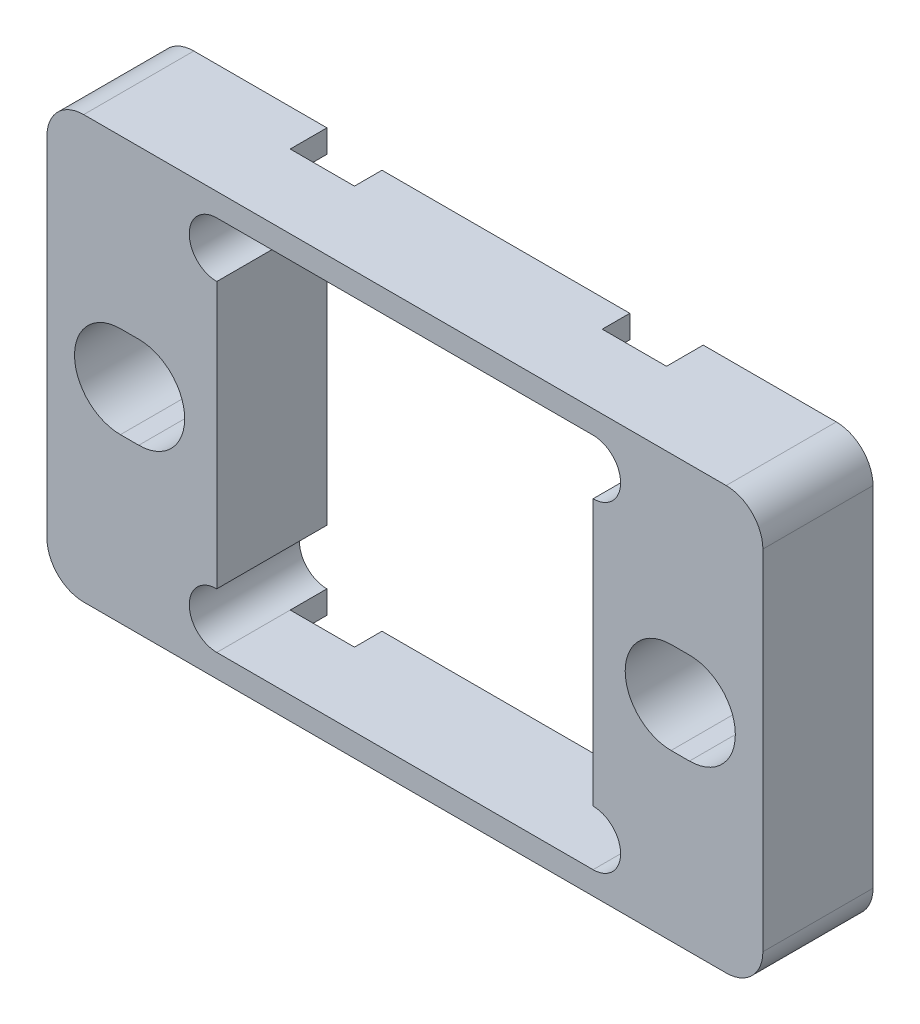
from build123d import *

# Parameters (mm, degrees)
SKETCH1_W           = 39
SKETCH1_H           = 23
SKETCH1_W_2         = 20.5
SKETCH1_H_2         = 20.5
BOSS_EXTRUDE1_DEPTH = 6
CUT_EXTRUDE1_REACH  = 32.745
SKETCH2_W           = 20.5
SKETCH2_H           = 4.35
SKETCH3_W           = 20.5
SKETCH3_H           = 1.25
BOSS_EXTRUDE2_DEPTH = 4.35
CUT_EXTRUDE2_REACH  = 32.745
CUT_EXTRUDE3_START  = -6
CUT_EXTRUDE3_DEPTH  = 6
CUT_EXTRUDE4_DEPTH  = 10
FILLET1_R           = 2


with BuildPart() as part:
    # Sketch1 → Boss-Extrude1 (new body)
    with BuildSketch(Plane.XY):
        Rectangle(SKETCH1_W, SKETCH1_H)
        Rectangle(SKETCH1_W_2, SKETCH1_H_2, mode=Mode.SUBTRACT)
    extrude(amount=BOSS_EXTRUDE1_DEPTH)

    # Cut-Extrude1: up to this face of the body (flat: up to its plane)
    cut_extrude1_end = Plane(part.part.faces().sort_by_distance((0, 11.5, 3))[0])
    # Sketch2 → Cut-Extrude1 (cut, up to the picked face)
    with BuildSketch(Plane.XZ.offset(11.5), mode=Mode.PRIVATE) as cut_extrude1_sk1:
        with Locations((0, 3.825)):
            Rectangle(SKETCH2_W, SKETCH2_H)
    cut_extrude1_tool1 = split(extrude(cut_extrude1_sk1.sketch, amount=-CUT_EXTRUDE1_REACH, mode=Mode.PRIVATE), bisect_by=cut_extrude1_end, keep=Keep.BOTH, mode=Mode.PRIVATE)
    add(cut_extrude1_tool1.solids().sort_by(Axis((0, -11.5, 3.825), (0, 1, 0)))[0], mode=Mode.SUBTRACT)

    # Sketch3 → Boss-Extrude2 (add)
    with BuildSketch(Plane.XY.offset(6)):
        with Locations((0, 10.875)):
            Rectangle(SKETCH3_W, SKETCH3_H)
        with Locations((0, -10.875)):
            Rectangle(SKETCH3_W, SKETCH3_H)
    extrude(amount=-BOSS_EXTRUDE2_DEPTH)

    # Cut-Extrude2: up to this face of the body (flat: up to its plane)
    cut_extrude2_end = Plane(part.part.faces().sort_by_distance((0, 11.5, 3))[0])
    # Sketch4 → Cut-Extrude2 (cut, up to the picked face)
    with BuildSketch(Plane.XZ.offset(11.5), mode=Mode.PRIVATE) as cut_extrude2_sk1:
        Polygon((6.75, 0.5), (6.75, 2), (10.25, 2), (10.25, 0), (6.75, 0), (-6.75, 0), (-10.25, 0), (-10.25, 2), (-6.75, 2), (-6.75, 0.5), align=None)
    cut_extrude2_tool1 = split(extrude(cut_extrude2_sk1.sketch, amount=-CUT_EXTRUDE2_REACH, mode=Mode.PRIVATE), bisect_by=cut_extrude2_end, keep=Keep.BOTH, mode=Mode.PRIVATE)
    add(cut_extrude2_tool1.solids().sort_by(Axis((6.955973, -11.5, 1.25), (0, 1, 0)))[0], mode=Mode.SUBTRACT)

    # Sketch5 → Cut-Extrude3 (cut)
    with BuildSketch(Plane(origin=(0, 0, 0), x_dir=(-1, 0, 0), z_dir=(0, 0, -1)).offset(CUT_EXTRUDE3_START)):
        with BuildLine():
            Line((-10.25, 10.25), (10.25, 10.25))
            ThreePointArc((10.25, 10.25), (11.75, 8.75), (10.25, 7.25))
            Line((10.25, 7.25), (-10.25, 7.25))
            ThreePointArc((-10.25, 7.25), (-11.75, 8.75), (-10.25, 10.25))
        make_face()
        with BuildLine():
            Line((-10.25, -7.25), (10.25, -7.25))
            ThreePointArc((10.25, -7.25), (11.75, -8.75), (10.25, -10.25))
            Line((10.25, -10.25), (-10.25, -10.25))
            ThreePointArc((-10.25, -10.25), (-11.75, -8.75), (-10.25, -7.25))
        make_face()
    extrude(amount=CUT_EXTRUDE3_DEPTH, mode=Mode.SUBTRACT)

    # Sketch6 → Cut-Extrude4 (cut)
    with BuildSketch(Plane.XY.offset(6)):
        with BuildLine():
            Line((-15.5, 2.4), (-14.5, 2.4))
            ThreePointArc((-14.5, 2.4), (-12, -0.1), (-14.5, -2.6))
            Line((-14.5, -2.6), (-15.5, -2.6))
            ThreePointArc((-15.5, -2.6), (-18, -0.1), (-15.5, 2.4))
        make_face()
        with BuildLine():
            Line((14.5, 2.5), (15.5, 2.5))
            ThreePointArc((15.5, 2.5), (18, 0), (15.5, -2.5))
            Line((15.5, -2.5), (14.5, -2.5))
            ThreePointArc((14.5, -2.5), (12, 0), (14.5, 2.5))
        make_face()
    extrude(amount=-CUT_EXTRUDE4_DEPTH, mode=Mode.SUBTRACT)

    # Fillet1
    fillet1_edges = [part.edges().sort_by_distance(p)[0] for p in [
        (19.5, -11.5, 3),
        (-19.5, -11.5, 3),
        (-19.5, 11.5, 3),
        (19.5, 11.5, 3),
    ]]
    fillet(fillet1_edges, radius=FILLET1_R)


solid = part.part
